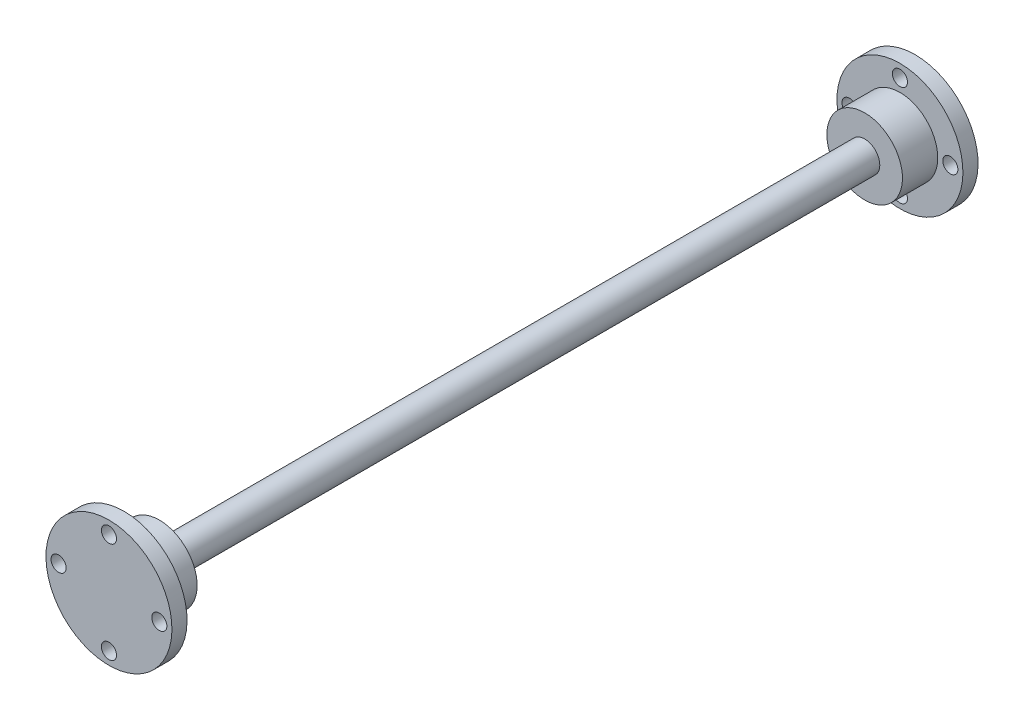
from build123d import *

# Parameters (mm, degrees)
SKETCH5_R          = 1.5
CUT_EXTRUDE4_DEPTH = 164


with BuildPart() as part:
    # Sketch4 → Revolve2 (revolve)
    with BuildSketch(Plane(origin=(0, 0, 0), x_dir=(0, 0, -1), z_dir=(1, 0, 0))):
        Polygon((-80, 0), (-80, 12.5), (-77, 12.5), (-77, 7.5), (-70, 7.5), (-70, 3), (0, 3), (0, 0), align=None)
    revolve2 = revolve(axis=Axis((0, 0, 0), (0, 0, 1)))

    # Mirror1: Revolve2 across plane
    add(revolve2.mirror(Plane(origin=(0, 0, 0), x_dir=(1, 0, 0), z_dir=(0, 0, -1))))

    # Sketch5 → Cut-Extrude4 (cut)
    with BuildSketch(Plane(origin=(0, 0, -80), x_dir=(-1, 0, 0), z_dir=(0, 0, -1))):
        with Locations(Location((10, 0, 0), (0, 0, 90))):
            Circle(SKETCH5_R)
        with Locations(Location((0, -10, 0), (0, 0, 90))):
            Circle(SKETCH5_R)
        with Locations(Location((-10, 0, 0), (0, 0, 90))):
            Circle(SKETCH5_R)
        with Locations(Location((0, 10, 0), (0, 0, 90))):
            Circle(SKETCH5_R)
    extrude(amount=-CUT_EXTRUDE4_DEPTH, mode=Mode.SUBTRACT)


solid = part.part
